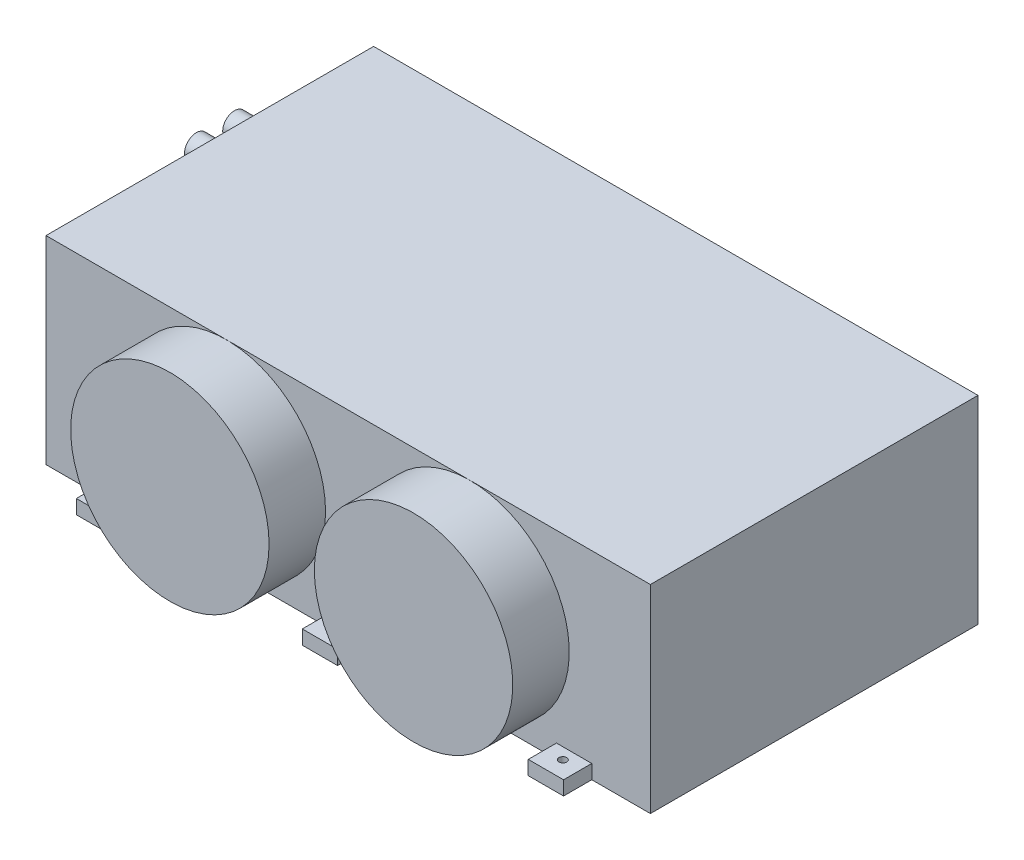
from build123d import *

# Parameters (mm, degrees)
SKETCH_1_W             = 856
SKETCH_1_H             = 464
EXTRUDE_1_DEPTH        = 281
SKETCH_3_W             = 50
SKETCH_3_H             = 40
EXTRUDE_2_DEPTH        = 20
PATTERN_LINEAR_2_COUNT = 2
PATTERN_LINEAR_2_PITCH = 320
SKETCH_4_R             = 5.5
CUT_EXTRUDE_1_DEPTH    = 571.341125994
SKETCH_5_R             = 140.5
EXTRUDE_3_DEPTH        = 80
SKETCH_6_R             = 16.75
SKETCH_6_R_2           = 13.25
EXTRUDE_4_DEPTH        = 34.5
PATTERN_LINEAR_3_COUNT = 2
PATTERN_LINEAR_3_PITCH = 54


with BuildPart() as part:
    # 草图1 → 凸台-拉伸1 (new body)
    with BuildSketch(Plane(origin=(0, 0, 0), x_dir=(1, 0, 0), z_dir=(0, 1, 0))):
        Rectangle(SKETCH_1_W, SKETCH_1_H)
    extrude(amount=EXTRUDE_1_DEPTH)


with BuildPart() as body_2:
    # 草图3 → 凸台-拉伸2 (new body)
    with BuildSketch(Plane.XZ):
        with Locations((0, 252)):
            Rectangle(SKETCH_3_W, SKETCH_3_H)
    extrude(amount=-EXTRUDE_2_DEPTH)


with BuildPart() as body_3:
    # 镜向1: mirrored copy
    add(body_2.part.mirror(Plane.XY))


with BuildPart() as pattern_linear_2_1:
    # 阵列(线性)2: pattern copy
    add(body_2.part.moved(Location(Vector(1, 0, 0) * (1 * PATTERN_LINEAR_2_PITCH))))


with BuildPart() as pattern_linear_2_2:
    # 阵列(线性)2: pattern copy
    add(body_3.part.moved(Location(Vector(1, 0, 0) * (1 * PATTERN_LINEAR_2_PITCH))))


with BuildPart() as body_6:
    # 镜向2: mirrored copy
    add(pattern_linear_2_1.part.mirror(Plane(origin=(0, 0, 0), x_dir=(0, 0, 1), z_dir=(1, 0, 0))))


with BuildPart() as body_7:
    # Mirror 2 2: mirrored copy
    add(pattern_linear_2_2.part.mirror(Plane(origin=(0, 0, 0), x_dir=(0, 0, 1), z_dir=(1, 0, 0))))


with BuildPart() as cut_extrude_1_tool:
    # 草图4 → 切除-拉伸1 (new, through all)
    with BuildSketch(Plane(origin=(0, 20, 0), x_dir=(1, 0, 0), z_dir=(0, 1, 0))):
        with Locations(Location((-320, 248, 0), (0, 0, 270))):
            Circle(SKETCH_4_R)
        with Locations(Location((0, 248, 0), (0, 0, 270))):
            Circle(SKETCH_4_R)
        with Locations(Location((320, 248, 0), (0, 0, 270))):
            Circle(SKETCH_4_R)
        with Locations(Location((0, -248, 0), (0, 0, 270))):
            Circle(SKETCH_4_R)
        with Locations(Location((320, -248, 0), (0, 0, 270))):
            Circle(SKETCH_4_R)
        with Locations(Location((-320, -248, 0), (0, 0, 270))):
            Circle(SKETCH_4_R)
    extrude(amount=-CUT_EXTRUDE_1_DEPTH)


with BuildPart() as body_2_1:
    add(body_2.part)

    # 切除-拉伸1: cut by cut_extrude_1_tool
    add(cut_extrude_1_tool.part, mode=Mode.SUBTRACT)


with BuildPart() as body_3_1:
    add(body_3.part)

    # 切除-拉伸1: cut by cut_extrude_1_tool
    add(cut_extrude_1_tool.part, mode=Mode.SUBTRACT)


with BuildPart() as pattern_linear_2_1_1:
    add(pattern_linear_2_1.part)

    # 切除-拉伸1: cut by cut_extrude_1_tool
    add(cut_extrude_1_tool.part, mode=Mode.SUBTRACT)


with BuildPart() as pattern_linear_2_2_1:
    add(pattern_linear_2_2.part)

    # 切除-拉伸1: cut by cut_extrude_1_tool
    add(cut_extrude_1_tool.part, mode=Mode.SUBTRACT)


with BuildPart() as body_6_1:
    add(body_6.part)

    # 切除-拉伸1: cut by cut_extrude_1_tool
    add(cut_extrude_1_tool.part, mode=Mode.SUBTRACT)


with BuildPart() as body_7_1:
    add(body_7.part)

    # 切除-拉伸1: cut by cut_extrude_1_tool
    add(cut_extrude_1_tool.part, mode=Mode.SUBTRACT)


with BuildPart() as body_8:
    # 草图5 → 凸台-拉伸3 (new body)
    with BuildSketch(Plane.XY.offset(232)):
        with Locations((-172.55753304, 140.5)):
            Circle(SKETCH_5_R)
    extrude(amount=EXTRUDE_3_DEPTH)


with BuildPart() as body_9:
    # 镜向3: mirrored copy
    add(body_8.part.mirror(Plane(origin=(0, 0, 0), x_dir=(0, 0, 1), z_dir=(1, 0, 0))))


with BuildPart() as body_10:
    # 草图6 → 凸台-拉伸4 (new body)
    with BuildSketch(Plane.ZY.offset(428)):
        with Locations((-69.5, 249.5)):
            Circle(SKETCH_6_R)
        with Locations((-69.5, 249.5)):
            Circle(SKETCH_6_R_2, mode=Mode.SUBTRACT)
    extrude(amount=EXTRUDE_4_DEPTH)


with BuildPart() as pattern_linear_3_1:
    # 阵列(线性)3: pattern copy
    add(body_10.part.moved(Location(Vector(0, 0, 1) * (1 * PATTERN_LINEAR_3_PITCH))))


solid = Compound([part.part, body_2_1.part, body_3_1.part, pattern_linear_2_1_1.part, pattern_linear_2_2_1.part, body_6_1.part, body_7_1.part, body_8.part, body_9.part, body_10.part, pattern_linear_3_1.part])
